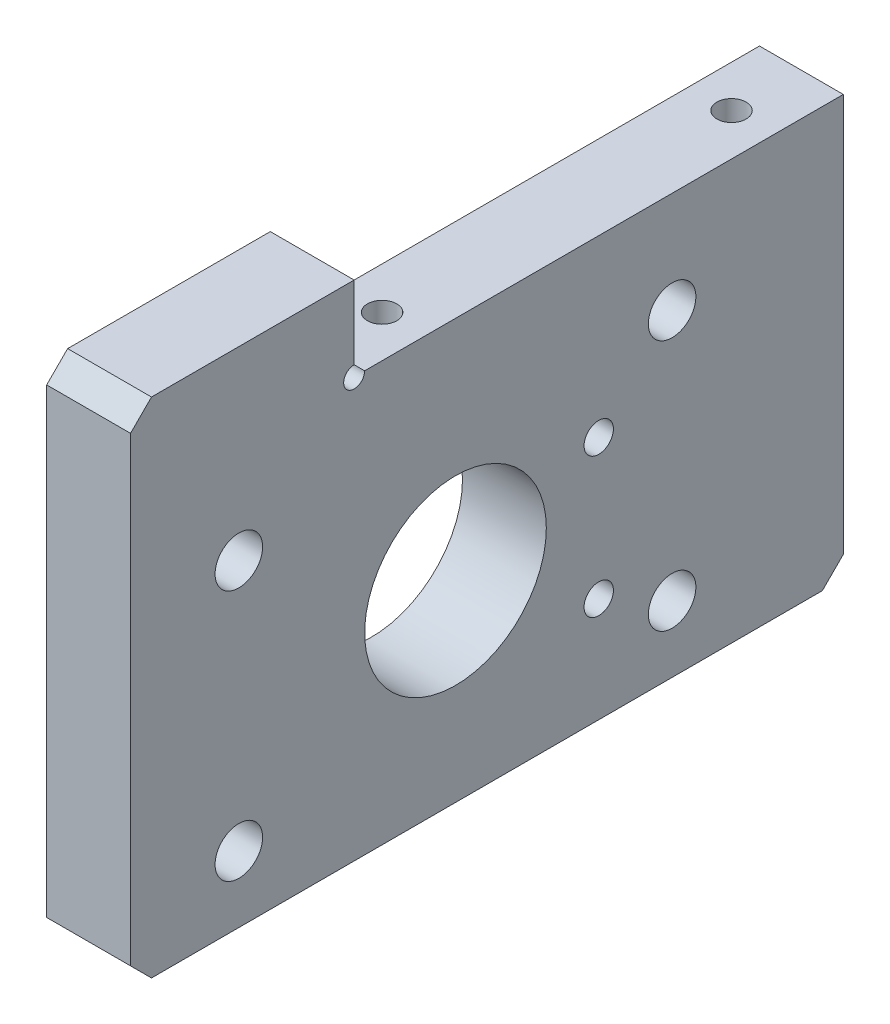
SolidWorks part; units mm, degrees
material "AL6061"
ref_plane "Front Plane" through (0, 0, 0) normal (0, 0, 1) x (1, 0, 0)
ref_plane "Top Plane" through (0, 0, 0) normal (0, 1, 0) x (1, 0, 0)
ref_plane "Right Plane" through (0, 0, 0) normal (1, 0, 0) x (0, 0, -1)
sketch "Sketch1" plane through (0, 0, 0) normal (1, 0, 0) x (0, 0, -1)
  line L0 (0, 0) -> (102, 0)
  line L1 (102, 0) -> (102, 60)
  line L2 (102, 60) -> (32, 60)
  line L3 (32, 60) -> (32, 72)
  line L4 (32, 72) -> (0, 72)
  line L5 (0, 72) -> (0, 0)
  dimension "D1" = 102
  dimension "D2" = 12
  dimension "D3" = 60
  dimension "D4" = 70
extrude "Boss-Extrude1" add sketch "Sketch1" along normal blind 12
sketch "Sketch2" plane through (12, 0, 0) normal (1, 0, 0) x (0, 0, -1)
  line L0 (0, 0) -> (102, 0) construction
  line L2 (46.5, 72) -> (46.5, 0) construction
  line L4 (0, 72) -> (0, 0) construction
  line L5 (32, 72) -> (0, 72) construction
  circle A0 centre (46.5, 27.5) radius 13
  dimension "D1" = 26
  dimension "D2" = 27.5
  dimension "D3" = 46.5
extrude "Cut-Extrude1" cut sketch "Sketch2" against normal through all
hole_wizard "M8 Tapped Hole1" positions "Sketch3" profile "Sketch4" tap size "M8" standard "GB"
sketch "Sketch3" plane through (0, 0, 0) normal (-1, 0, 0) x (0, 0, 1)
  point P0 (-77.5, 45.5)
  point P3 (-77.5, 9.5)
  point P6 (-15.5, 9.5)
  point P9 (-15.5, 45.5)
sketch "Sketch4" plane through (0, 45.5, -77.5) normal (0, 1, 0) x (0, 0, 1)
  line L0 (0, 0) -> (0, 21.7929)
  line L1 (0, 21.7929) -> (3.4, 19.75)
  line L2 (3.4, 19.75) -> (3.4, 0)
  line L5 (3.4, 0) -> (0, 0)
  line L10 (0, 21.7929) -> (-3.4, 19.75) construction
  line L11 (0, -6.35) -> (0, 107.95) construction
  dimension "螺纹孔钻头直径" = 6.8
  dimension "螺纹孔钻头深度" = 19.75
  dimension "导头角度" = 118
cosmetic thread "Cosmetic Thread3" parameters "D1"=16, "D2"=8
cosmetic thread "Cosmetic Thread9" parameters "D1"=16, "D2"=8
cosmetic thread "Cosmetic Thread10" parameters "D1"=16, "D2"=8
cosmetic thread "Cosmetic Thread12" parameters "D1"=16, "D2"=8
hole_wizard "M5 Tapped Hole1" positions "Sketch7" profile "Sketch8" tap size "M5" standard "GB"
sketch "Sketch7" plane through (12, 0, 0) normal (1, 0, 0) x (0, 0, -1)
  point P0 (67, 35)
  point P3 (67, 15)
sketch "Sketch8" plane through (12, 35, -67) normal (0, 1, 0) x (0, 0, -1)
  line L0 (0, 0) -> (0, 13.6618)
  line L1 (0, 13.6618) -> (2.1, 12.4)
  line L2 (2.1, 12.4) -> (2.1, 0)
  line L5 (2.1, 0) -> (0, 0)
  line L10 (0, 13.6618) -> (-2.1, 12.4) construction
  line L11 (0, -6.35) -> (0, 107.95) construction
  dimension "螺纹孔钻头直径" = 4.2
  dimension "螺纹孔钻头深度" = 12.4
  dimension "导头角度" = 118
cosmetic thread "Cosmetic Thread5" parameters "D1"=10, "D2"=5
cosmetic thread "Cosmetic Thread11" parameters "D1"=10, "D2"=5
hole_wizard "M5 Tapped Hole2" positions "Sketch9" profile "Sketch10" tap size "M5" standard "GB"
sketch "Sketch9" plane through (0, 60, 0) normal (0, 1, 0) x (1, 0, 0)
  line L0 (6, 102) -> (6, 32) construction
  line L1 (12, 102) -> (0, 102) construction
  line L2 (12, 32) -> (0, 32) construction
  line L4 (12, 67) -> (0, 67) construction
  line L5 (12, 102) -> (12, 32) construction
  line L6 (0, 102) -> (0, 32) construction
  point P17 (6, 92)
  point P19 (6, 42)
  dimension "D1" = 50
sketch "Sketch10" plane through (6, 60, -42) normal (1, 0, 0) x (0, 0, 1)
  line L0 (0, 0) -> (0, 13.6618)
  line L1 (0, 13.6618) -> (2.1, 12.4)
  line L2 (2.1, 12.4) -> (2.1, 0)
  line L5 (2.1, 0) -> (0, 0)
  line L10 (0, 13.6618) -> (-2.1, 12.4) construction
  line L11 (0, -6.35) -> (0, 107.95) construction
  dimension "螺纹孔钻头直径" = 4.2
  dimension "螺纹孔钻头深度" = 12.4
  dimension "导头角度" = 118
cosmetic thread "Cosmetic Thread7" parameters "D1"=10, "D2"=5
cosmetic thread "Cosmetic Thread8" parameters "D1"=10, "D2"=5
chamfer "Chamfer1" distance 3 angle 45 3 edges at (6, 72, 0) (6, 0, -102) (6, 0, 0)
sketch "Sketch11" plane through (12, 0, 0) normal (1, 0, 0) x (0, 0, -1)
  circle A0 centre (32, 60) radius 1.5
  dimension "D1" = 3
extrude "Cut-Extrude2" cut sketch "Sketch11" against normal through all
